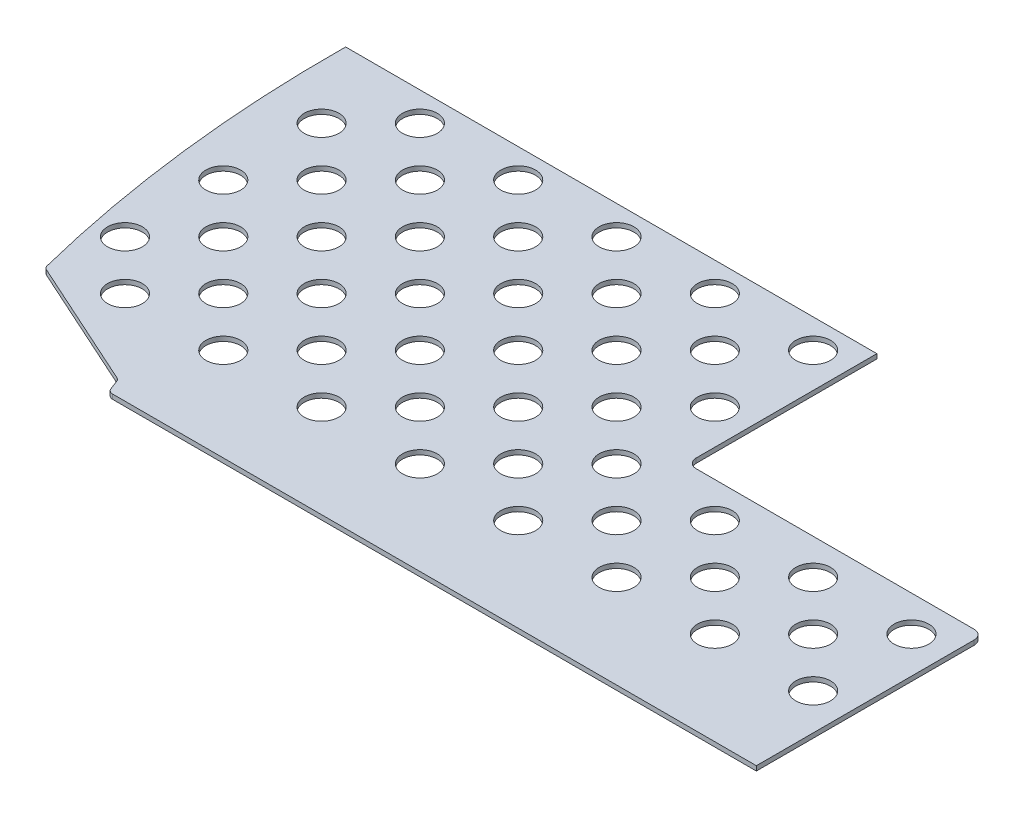
from build123d import *

# Parameters (mm, degrees)
SKETCH1_R           = 15
BOSS_EXTRUDE1_DEPTH = 4


with BuildPart() as part:
    # Sketch1 → Boss-Extrude1 (new body)
    with BuildSketch(Plane.XZ):
        with BuildLine():
            Line((119.63460713, -7.226728829), (116.577483445, -15.286418544))
            ThreePointArc((116.577483445, -15.286418544), (115.546776451, -16.936481806), (113.964315794, -18.068243242))
            Line((113.964315794, -18.068243242), (3.00769119, -68.291683558))
            ThreePointArc((3.00769119, -68.291683558), (1.232907358, -69.640462039), (0.220696267, -71.626535993))
            ThreePointArc((0.220696267, -71.626535993), (-26.539465951, -216.697676507), (-34.524926809, -364))
            Line((-34.524926809, -364), (423.975073191, -364))
            Line((423.975073191, -364), (423.975073191, -208))
            ThreePointArc((423.975073191, -208), (426.318218942, -202.343145751), (431.975073191, -200))
            Line((431.975073191, -200), (671.975073191, -200))
            ThreePointArc((671.975073191, -200), (677.63192744, -197.656854249), (679.975073191, -192))
            Line((679.975073191, -192), (679.975073191, -4))
            Line((679.975073191, -4), (124.309594762, -4))
            ThreePointArc((124.309594762, -4), (121.469379616, -4.885005719), (119.63460713, -7.226728829))
        make_face()
        with Locations(Location((393.975073191, -254.147186258, 0), (0, 0, 90))):
            Circle(SKETCH1_R, mode=Mode.SUBTRACT)
        with Locations(Location((351.54866632, -296.573593129, 0), (0, 0, 90))):
            Circle(SKETCH1_R, mode=Mode.SUBTRACT)
        with Locations(Location((309.122259449, -339, 0), (0, 0, 90))):
            Circle(SKETCH1_R, mode=Mode.SUBTRACT)
        with Locations(Location((393.975073191, -169.294372515, 0), (0, 0, 90))):
            Circle(SKETCH1_R, mode=Mode.SUBTRACT)
        with Locations(Location((351.54866632, -211.720779386, 0), (0, 0, 90))):
            Circle(SKETCH1_R, mode=Mode.SUBTRACT)
        with Locations(Location((309.122259449, -254.147186258, 0), (0, 0, 90))):
            Circle(SKETCH1_R, mode=Mode.SUBTRACT)
        with Locations(Location((266.695852577, -296.573593129, 0), (0, 0, 90))):
            Circle(SKETCH1_R, mode=Mode.SUBTRACT)
        with Locations(Location((224.269445706, -339, 0), (0, 0, 90))):
            Circle(SKETCH1_R, mode=Mode.SUBTRACT)
        with Locations(Location((478.827886933, -169.294372515, 0), (0, 0, 90))):
            Circle(SKETCH1_R, mode=Mode.SUBTRACT)
        with Locations(Location((436.401480062, -126.867965644, 0), (0, 0, 90))):
            Circle(SKETCH1_R, mode=Mode.SUBTRACT)
        with Locations(Location((393.975073191, -84.441558773, 0), (0, 0, 90))):
            Circle(SKETCH1_R, mode=Mode.SUBTRACT)
        with Locations(Location((351.54866632, -126.867965644, 0), (0, 0, 90))):
            Circle(SKETCH1_R, mode=Mode.SUBTRACT)
        with Locations(Location((309.122259449, -169.294372515, 0), (0, 0, 90))):
            Circle(SKETCH1_R, mode=Mode.SUBTRACT)
        with Locations(Location((266.695852577, -211.720779386, 0), (0, 0, 90))):
            Circle(SKETCH1_R, mode=Mode.SUBTRACT)
        with Locations(Location((224.269445706, -254.147186258, 0), (0, 0, 90))):
            Circle(SKETCH1_R, mode=Mode.SUBTRACT)
        with Locations(Location((181.843038835, -296.573593129, 0), (0, 0, 90))):
            Circle(SKETCH1_R, mode=Mode.SUBTRACT)
        with Locations(Location((139.416631964, -339, 0), (0, 0, 90))):
            Circle(SKETCH1_R, mode=Mode.SUBTRACT)
        with Locations(Location((563.680700676, -169.294372515, 0), (0, 0, 90))):
            Circle(SKETCH1_R, mode=Mode.SUBTRACT)
        with Locations(Location((521.254293805, -126.867965644, 0), (0, 0, 90))):
            Circle(SKETCH1_R, mode=Mode.SUBTRACT)
        with Locations(Location((478.827886933, -84.441558773, 0), (0, 0, 90))):
            Circle(SKETCH1_R, mode=Mode.SUBTRACT)
        with Locations(Location((309.122259449, -84.441558773, 0), (0, 0, 90))):
            Circle(SKETCH1_R, mode=Mode.SUBTRACT)
        with Locations(Location((266.695852577, -126.867965644, 0), (0, 0, 90))):
            Circle(SKETCH1_R, mode=Mode.SUBTRACT)
        with Locations(Location((224.269445706, -169.294372515, 0), (0, 0, 90))):
            Circle(SKETCH1_R, mode=Mode.SUBTRACT)
        with Locations(Location((181.843038835, -211.720779386, 0), (0, 0, 90))):
            Circle(SKETCH1_R, mode=Mode.SUBTRACT)
        with Locations(Location((139.416631964, -254.147186258, 0), (0, 0, 90))):
            Circle(SKETCH1_R, mode=Mode.SUBTRACT)
        with Locations(Location((96.990225093, -296.573593129, 0), (0, 0, 90))):
            Circle(SKETCH1_R, mode=Mode.SUBTRACT)
        with Locations(Location((54.563818221, -339, 0), (0, 0, 90))):
            Circle(SKETCH1_R, mode=Mode.SUBTRACT)
        with Locations(Location((648.533514418, -169.294372515, 0), (0, 0, 90))):
            Circle(SKETCH1_R, mode=Mode.SUBTRACT)
        with Locations(Location((606.107107547, -126.867965644, 0), (0, 0, 90))):
            Circle(SKETCH1_R, mode=Mode.SUBTRACT)
        with Locations(Location((563.680700676, -84.441558773, 0), (0, 0, 90))):
            Circle(SKETCH1_R, mode=Mode.SUBTRACT)
        with Locations(Location((224.269445706, -84.441558773, 0), (0, 0, 90))):
            Circle(SKETCH1_R, mode=Mode.SUBTRACT)
        with Locations(Location((181.843038835, -126.867965644, 0), (0, 0, 90))):
            Circle(SKETCH1_R, mode=Mode.SUBTRACT)
        with Locations(Location((139.416631964, -169.294372515, 0), (0, 0, 90))):
            Circle(SKETCH1_R, mode=Mode.SUBTRACT)
        with Locations(Location((96.990225093, -211.720779386, 0), (0, 0, 90))):
            Circle(SKETCH1_R, mode=Mode.SUBTRACT)
        with Locations(Location((54.563818221, -254.147186258, 0), (0, 0, 90))):
            Circle(SKETCH1_R, mode=Mode.SUBTRACT)
        with Locations(Location((12.13741135, -296.573593129, 0), (0, 0, 90))):
            Circle(SKETCH1_R, mode=Mode.SUBTRACT)
        with Locations(Location((648.533514418, -84.441558773, 0), (0, 0, 90))):
            Circle(SKETCH1_R, mode=Mode.SUBTRACT)
        with Locations(Location((139.416631964, -84.441558773, 0), (0, 0, 90))):
            Circle(SKETCH1_R, mode=Mode.SUBTRACT)
        with Locations(Location((96.990225093, -126.867965644, 0), (0, 0, 90))):
            Circle(SKETCH1_R, mode=Mode.SUBTRACT)
        with Locations(Location((54.563818221, -169.294372515, 0), (0, 0, 90))):
            Circle(SKETCH1_R, mode=Mode.SUBTRACT)
        with Locations(Location((12.13741135, -211.720779386, 0), (0, 0, 90))):
            Circle(SKETCH1_R, mode=Mode.SUBTRACT)
        with Locations(Location((54.563818221, -84.441558773, 0), (0, 0, 90))):
            Circle(SKETCH1_R, mode=Mode.SUBTRACT)
        with Locations(Location((12.13741135, -126.867965644, 0), (0, 0, 90))):
            Circle(SKETCH1_R, mode=Mode.SUBTRACT)
        with Locations(Location((393.975073191, -339, 0), (0, 0, 90))):
            Circle(SKETCH1_R, mode=Mode.SUBTRACT)
    extrude(amount=-BOSS_EXTRUDE1_DEPTH)


solid = part.part
